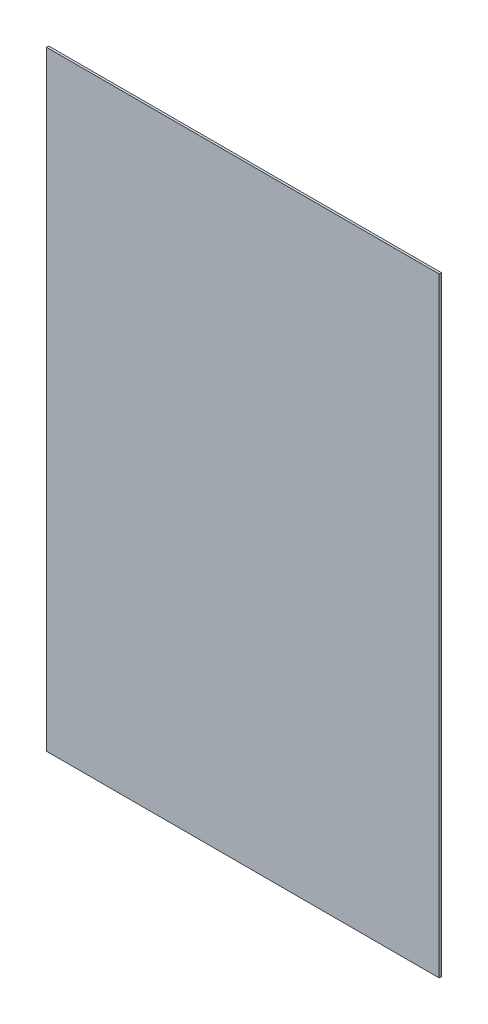
from build123d import *

# Parameters (mm, degrees)
SKETCH_1_W      = 876
SKETCH_1_H      = 1360
EXTRUDE_1_DEPTH = 5


with BuildPart() as part:
    # 草图1 → 凸台-拉伸1 (new body)
    with BuildSketch(Plane.XY):
        Rectangle(SKETCH_1_W, SKETCH_1_H)
    extrude(amount=EXTRUDE_1_DEPTH)


solid = part.part
